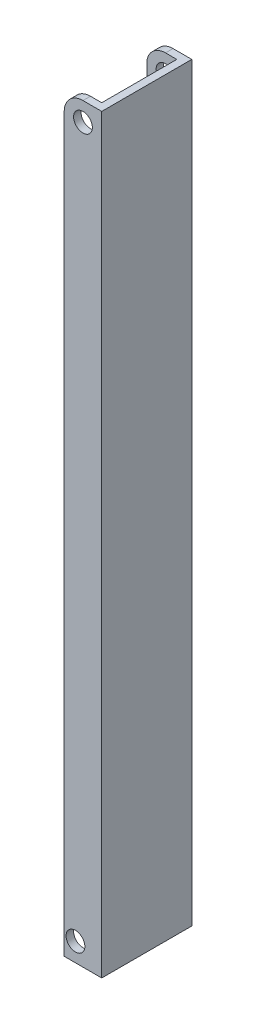
from build123d import *

# Parameters (mm, degrees)
BOSS_EXTRUDE1_DEPTH     = 200
CUT_EXTRUDE1_DEPTH      = 254.860197747
CUT_EXTRUDE1_DEPTH_BACK = 254.860197747
SKETCH3_R               = 2.5
FILLET1_R               = 5
CUT_EXTRUDE2_DEPTH      = 254.860197747
CUT_EXTRUDE2_DEPTH_BACK = 254.860197747
SKETCH5_R               = 2.5


with BuildPart() as part:
    # Sketch2 → Boss-Extrude1 (new body)
    with BuildSketch(Plane(origin=(0, 50, 0), x_dir=(1, 0, 0), z_dir=(0, 1, 0))):
        Polygon((35, 10), (35, 20), (27, 20), (27, 22), (37, 22), (37, -2), (27, -2), (27, 0), (35, 0), align=None)
    extrude(amount=BOSS_EXTRUDE1_DEPTH)

    # Sketch3 → Cut-Extrude1 (cut, two sides: drawn at the far end of the back side and taken through both)
    with BuildSketch(Plane.XY.offset(2).offset(-CUT_EXTRUDE1_DEPTH_BACK)):
        with Locations((30, 55)):
            Circle(SKETCH3_R)
    extrude(amount=CUT_EXTRUDE1_DEPTH + CUT_EXTRUDE1_DEPTH_BACK, mode=Mode.SUBTRACT)

    # Fillet1
    fillet1_edges = [part.edges().sort_by_distance(p)[0] for p in [
        (27, 250, 1),
        (27, 250, -21),
    ]]
    fillet(fillet1_edges, radius=FILLET1_R)

    # Sketch5 → Cut-Extrude2 (cut, two sides: drawn at the far end of the back side and taken through both)
    with BuildSketch(Plane.XY.offset(2).offset(-CUT_EXTRUDE2_DEPTH_BACK)):
        with Locations((32, 245)):
            Circle(SKETCH5_R)
    extrude(amount=CUT_EXTRUDE2_DEPTH + CUT_EXTRUDE2_DEPTH_BACK, mode=Mode.SUBTRACT)


solid = part.part
